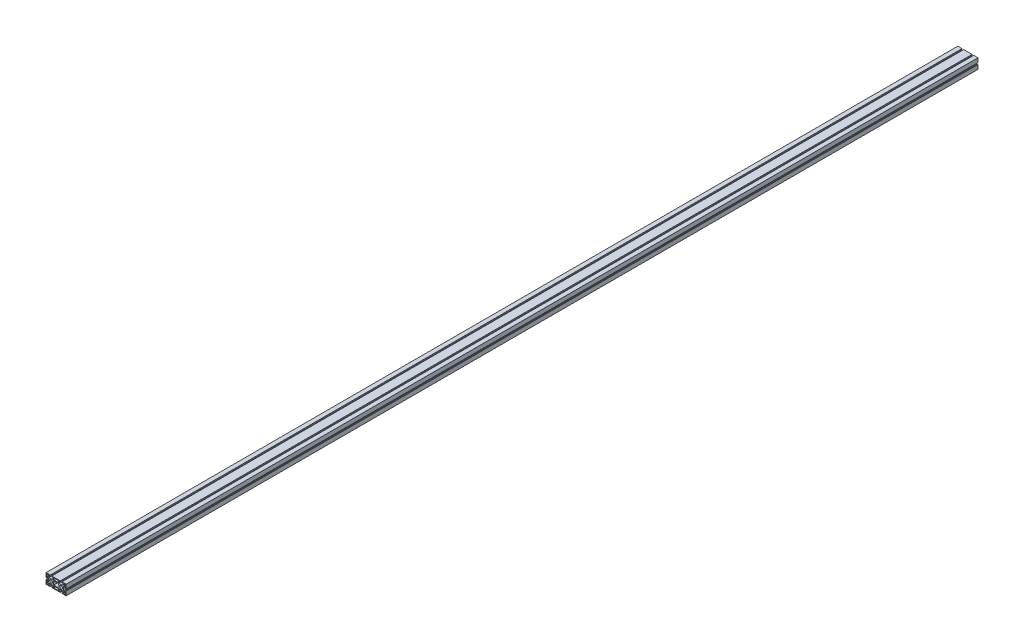
SolidWorks part; units mm, degrees
ref_plane "前视基准面" through (0, 0, 0) normal (0, 0, 1) x (1, 0, 0)
ref_plane "上视基准面" through (0, 0, 0) normal (0, 1, 0) x (1, 0, 0)
ref_plane "右视基准面" through (0, 0, 0) normal (1, 0, 0) x (0, 0, -1)
sketch "草图1" plane through (0, 0, 0) normal (0, 0, 1) x (1, 0, 0)
  line L0 (12.5, 0) -> (12.5, -2)
  line L1 (0, 0) -> (12.5, 0)
  line L2 (0, 0) -> (0, -12.5)
  line L3 (0, -30) -> (12.5, -30)
  line L4 (30, 0) -> (30, -30) construction
  line L5 (17.5, 0) -> (17.5, -2)
  line L6 (12.5, -2) -> (9.5, -2)
  line L7 (9.5, -2) -> (9.5, -7)
  line L8 (17.5, -2) -> (20.5, -2)
  line L9 (20.5, -2) -> (20.5, -7)
  line L10 (0, -15) -> (30, -15) construction
  line L11 (9.5, -28) -> (9.5, -23)
  line L12 (12.5, -28) -> (9.5, -28)
  line L13 (12.5, -30) -> (12.5, -28)
  line L14 (17.5, -30) -> (17.5, -28)
  line L15 (17.5, -28) -> (20.5, -28)
  line L16 (20.5, -28) -> (20.5, -23)
  line L17 (0, -17.5) -> (2, -17.5)
  line L18 (2, -20.5) -> (7, -20.5)
  line L19 (2, -9.5) -> (7, -9.5)
  line L20 (2, -12.5) -> (2, -9.5)
  line L21 (2, -17.5) -> (2, -20.5)
  line L22 (0, -12.5) -> (2, -12.5)
  line L23 (32, -12.5) -> (28, -12.5)
  line L24 (28, -9.5) -> (23, -9.5)
  line L25 (28, -20.5) -> (23, -20.5)
  line L26 (28, -17.5) -> (28, -20.5)
  line L27 (28, -12.5) -> (28, -9.5)
  line L28 (32, -17.5) -> (28, -17.5)
  line L29 (17.5, 0) -> (42.5, 0)
  line L30 (0, -17.5) -> (0, -30)
  line L31 (53, -2) -> (53, -7)
  line L32 (17.5, -30) -> (42.5, -30)
  line L33 (23, -23) -> (28, -23)
  line L34 (23, -2) -> (28, -2)
  line L35 (23, -2) -> (23, -7)
  line L36 (23, -7) -> (28, -7)
  line L37 (28, -2) -> (28, -7)
  line L38 (28, -28) -> (28, -23)
  line L39 (23, -28) -> (28, -28)
  line L40 (23, -28) -> (23, -23)
  line L41 (15, -33.907) -> (15, 0) construction
  line L42 (7, -28) -> (2, -28)
  line L43 (7, -28) -> (7, -23)
  line L44 (2, -28) -> (2, -23)
  line L45 (7, -23) -> (2, -23)
  line L46 (7, -7) -> (2, -7)
  line L47 (2, -2) -> (2, -7)
  line L48 (7, -2) -> (2, -2)
  line L49 (7, -2) -> (7, -7)
  line L50 (53, -2) -> (58, -2)
  line L51 (58, -2) -> (58, -7)
  line L52 (53, -7) -> (58, -7)
  line L53 (53, -23) -> (58, -23)
  line L54 (58, -28) -> (58, -23)
  line L55 (53, -28) -> (53, -23)
  line L56 (53, -28) -> (58, -28)
  line L57 (60, -17.5) -> (60, -30)
  line L58 (60, -12.5) -> (58, -12.5)
  line L59 (58, -17.5) -> (58, -20.5)
  line L60 (58, -12.5) -> (58, -9.5)
  line L61 (58, -9.5) -> (53, -9.5)
  line L62 (58, -20.5) -> (53, -20.5)
  line L63 (60, -17.5) -> (58, -17.5)
  line L64 (47.5, -30) -> (47.5, -28)
  line L65 (47.5, -28) -> (50.5, -28)
  line L66 (50.5, -28) -> (50.5, -23)
  line L67 (50.5, -2) -> (50.5, -7)
  line L68 (47.5, -2) -> (50.5, -2)
  line L69 (60, -30) -> (47.5, -30)
  line L70 (60, 0) -> (60, -12.5)
  line L71 (60, 0) -> (47.5, 0)
  line L72 (47.5, 0) -> (47.5, -2)
  line L73 (37, -28) -> (37, -23)
  line L74 (37, -28) -> (32, -28)
  line L75 (32, -28) -> (32, -23)
  line L76 (32, -2) -> (32, -7)
  line L77 (37, -7) -> (32, -7)
  line L78 (37, -2) -> (37, -7)
  line L79 (37, -2) -> (32, -2)
  line L80 (37, -23) -> (32, -23)
  line L81 (32, -12.5) -> (32, -9.5)
  line L82 (32, -17.5) -> (32, -20.5)
  line L83 (32, -20.5) -> (37, -20.5)
  line L84 (32, -9.5) -> (37, -9.5)
  line L85 (39.5, -28) -> (39.5, -23)
  line L86 (42.5, -28) -> (39.5, -28)
  line L87 (42.5, -30) -> (42.5, -28)
  line L88 (39.5, -2) -> (39.5, -7)
  line L89 (42.5, -2) -> (39.5, -2)
  line L90 (42.5, 0) -> (42.5, -2)
  arc A0 (9.5, -7) -> (20.5, -7) centre (15, 3.907) ccw
  arc A1 (9.5, -23) -> (20.5, -23) centre (15, -33.907) cw
  arc A2 (7, -20.5) -> (7, -9.5) centre (-3.907, -15) ccw
  arc A3 (23, -9.5) -> (23, -20.5) centre (33.907, -15) ccw
  circle A4 centre (15, -15) radius 4.1077
  arc A5 (50.5, -23) -> (39.5, -23) centre (45, -33.907) ccw
  arc A6 (50.5, -7) -> (39.5, -7) centre (45, 3.907) cw
  circle A7 centre (45, -15) radius 4.1077
  arc A8 (53, -20.5) -> (53, -9.5) centre (63.907, -15) cw
  arc A9 (37, -9.5) -> (37, -20.5) centre (26.093, -15) cw
  point P107 (30, -17.5)
  point P110 (30, -12.5)
  dimension "D6" = 12.2153
  dimension "D1" = 5
  dimension "D2" = 12.5
  dimension "D3" = 2
  dimension "D4" = 3
  dimension "D5" = 5
  dimension "D7" = 30
  dimension "D8" = 30
  dimension "D9" = 2.5
  dimension "D10" = 2.5
  dimension "D11" = 5
  dimension "D12" = 5
  dimension "D13" = 5
  dimension "D14" = 2
  dimension "D15" = 12.5
  dimension "D16" = 5
  dimension "D17" = 3
  dimension "D18" = 2
  dimension "D19" = 3
extrude "拉伸1" add sketch "草图1" along normal blind 2720
sketch "草图2" plane through (0, 0, 2720) normal (0, 0, 1) x (1, 0, 0)
  line L1 (28, -2) -> (32, -2)
  line L2 (28, -2) -> (28, -7)
  line L3 (28, -7) -> (32, -7)
  line L4 (32, -2) -> (32, -7)
  line L5 (28, -23) -> (32, -23)
  line L6 (28, -23) -> (28, -28)
  line L7 (28, -28) -> (32, -28)
  line L8 (32, -23) -> (32, -28)
extrude "切除-拉伸1" cut sketch "草图2" against normal through all
sketch "草图3" plane through (0, 0, 2720) normal (0, 0, 1) x (1, 0, 0)
  line L1 (28, -9.5) -> (32, -9.5)
  line L2 (28, -9.5) -> (28, -20.5)
  line L3 (28, -20.5) -> (32, -20.5)
  line L4 (32, -9.5) -> (32, -20.5)
extrude "切除-拉伸2" cut sketch "草图3" against normal through all
